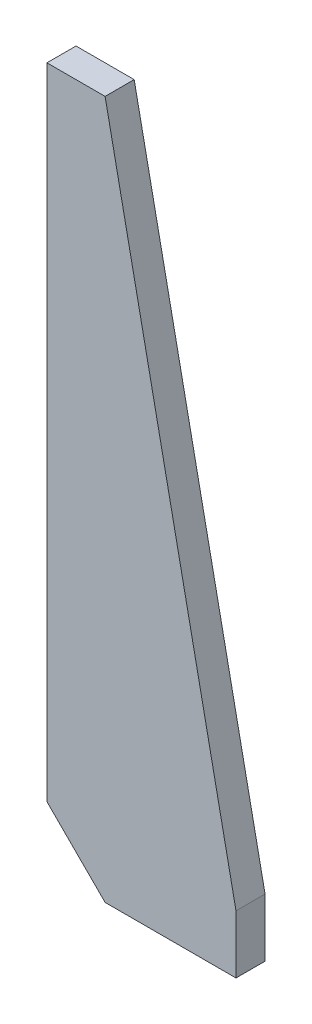
from build123d import *

# Parameters (mm, degrees)
BOSS_EXTRUDE1_DEPTH = 5
CHAMFER1_SIZE       = 20


with BuildPart() as part:
    # Sketch1 → Boss-Extrude1 (new, symmetric)
    with BuildSketch(Plane.XY):
        Polygon((0, 0), (65, 0), (65, 20), (20, 240), (0, 240), align=None)
    extrude(amount=BOSS_EXTRUDE1_DEPTH, both=True)

    # Chamfer1
    chamfer1_edges = [part.edges().sort_by_distance(p)[0] for p in [
        (0, 0, 0),
    ]]
    chamfer(chamfer1_edges, length=CHAMFER1_SIZE)


solid = part.part
